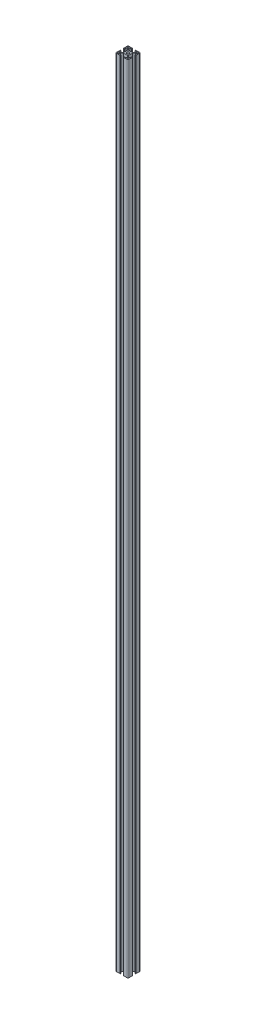
from build123d import *

# Parameters (mm, degrees)
SKETCH_1_R                = 2.1
SKETCH_1_R_2              = 3.4
EXTRUDE_1_DEPTH           = 1940
HOLE_WIZARD_1_D           = 6.6
HOLE_WIZARD_1_CBORE_D     = 11
HOLE_WIZARD_1_CBORE_DEPTH = 9


with BuildPart() as part:
    # 草图1 → 拉伸1 (new body)
    with BuildSketch(Plane(origin=(0, 0, 0), x_dir=(1, 0, 0), z_dir=(0, 1, 0))):
        with BuildLine():
            Line((6.75, -28), (11, -28))
            Line((11, -28), (11, -30))
            Line((11, -30), (2, -30))
            ThreePointArc((2, -30), (0.585786438, -29.414213562), (0, -28))
            Line((0, -28), (0, -19))
            Line((0, -19), (2, -19))
            Line((2, -19), (2, -23.25))
            Line((2, -23.25), (5.335785999, -23.25))
            Line((5.335785999, -23.25), (9, -19.585785999))
            Line((9, -19.585785999), (9, -10.414214001))
            Line((9, -10.414214001), (5.335785999, -6.75))
            Line((5.335785999, -6.75), (2, -6.75))
            Line((2, -6.75), (2, -11))
            Line((2, -11), (0, -11))
            Line((0, -11), (0, -2))
            ThreePointArc((0, -2), (0.585786438, -0.585786438), (2, 0))
            Line((2, 0), (11, 0))
            Line((11, 0), (11, -2))
            Line((11, -2), (6.75, -2))
            Line((6.75, -2), (6.75, -5.335785999))
            Line((6.75, -5.335785999), (10.414214001, -9))
            Line((10.414214001, -9), (19.585785999, -9))
            Line((19.585785999, -9), (23.25, -5.335785999))
            Line((23.25, -5.335785999), (23.25, -2))
            Line((23.25, -2), (19, -2))
            Line((19, -2), (19, 0))
            Line((19, 0), (28, 0))
            ThreePointArc((28, 0), (29.414213562, -0.585786438), (30, -2))
            Line((30, -2), (30, -11))
            Line((30, -11), (28, -11))
            Line((28, -11), (28, -6.75))
            Line((28, -6.75), (24.664214001, -6.75))
            Line((24.664214001, -6.75), (21, -10.414214001))
            Line((21, -10.414214001), (21, -19.585785999))
            Line((21, -19.585785999), (24.664214001, -23.25))
            Line((24.664214001, -23.25), (28, -23.25))
            Line((28, -23.25), (28, -19))
            Line((28, -19), (30, -19))
            Line((30, -19), (30, -28))
            ThreePointArc((30, -28), (29.414213562, -29.414213562), (28, -30))
            Line((28, -30), (19, -30))
            Line((19, -30), (19, -28))
            Line((19, -28), (23.25, -28))
            Line((23.25, -28), (23.25, -24.664214001))
            Line((23.25, -24.664214001), (19.585785999, -21))
            Line((19.585785999, -21), (10.414214001, -21))
            Line((10.414214001, -21), (6.75, -24.664214001))
            Line((6.75, -24.664214001), (6.75, -28))
        make_face()
        with Locations(Location((3.375, -26.625, 0), (0, 0, 270))):
            Circle(SKETCH_1_R, mode=Mode.SUBTRACT)
        with Locations(Location((26.625, -26.625, 0), (0, 0, 270))):
            Circle(SKETCH_1_R, mode=Mode.SUBTRACT)
        with Locations(Location((15, -15, 0), (0, 0, 270))):
            Circle(SKETCH_1_R_2, mode=Mode.SUBTRACT)
        with Locations(Location((3.375, -3.375, 0), (0, 0, 270))):
            Circle(SKETCH_1_R, mode=Mode.SUBTRACT)
        with Locations(Location((26.625, -3.375, 0), (0, 0, 270))):
            Circle(SKETCH_1_R, mode=Mode.SUBTRACT)
    extrude(amount=EXTRUDE_1_DEPTH)

    # 打孔尺寸根据内六角圆柱头螺钉的类型1 (through all)
    with Locations(Plane.ZY):
        with Locations((15, 70), (15, 1870), (15, 1270), (15, 670)):
            CounterBoreHole(HOLE_WIZARD_1_D / 2, HOLE_WIZARD_1_CBORE_D / 2, HOLE_WIZARD_1_CBORE_DEPTH)


solid = part.part
